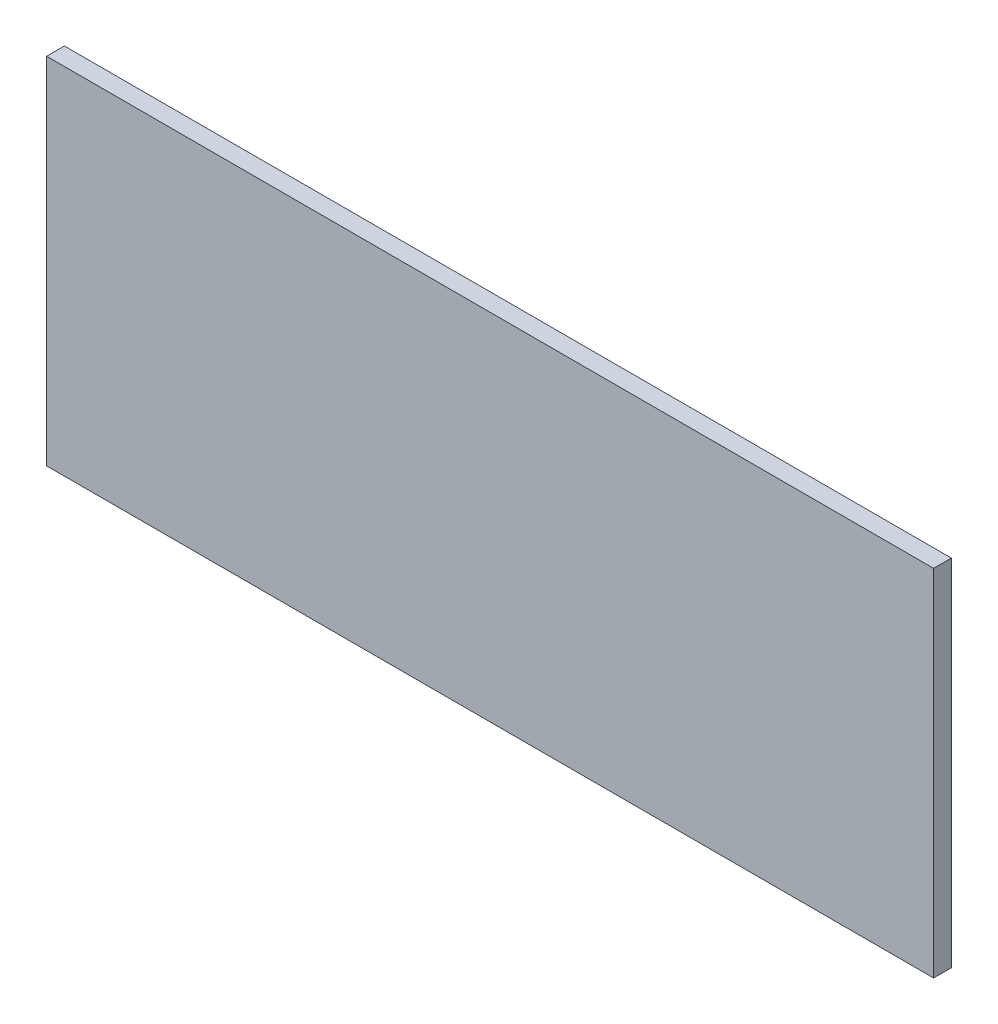
SolidWorks part; units mm, degrees
ref_plane "Front Plane" through (0, 0, 0) normal (0, 0, 1) x (1, 0, 0)
ref_plane "Top Plane" through (0, 0, 0) normal (0, 1, 0) x (1, 0, 0)
ref_plane "Right Plane" through (0, 0, 0) normal (1, 0, 0) x (0, 0, -1)
sketch "Sketch1" plane through (0, 0, 0) normal (0, 0, 1) x (1, 0, 0)
  line L1 (0, 0) -> (5000, 0)
  line L2 (0, 0) -> (0, 2000)
  line L3 (0, 2000) -> (5000, 2000)
  line L4 (5000, 0) -> (5000, 2000)
  dimension "D1" = 2000
  dimension "D2" = 5000
extrude "Boss-Extrude1" add sketch "Sketch1" along normal blind 100
